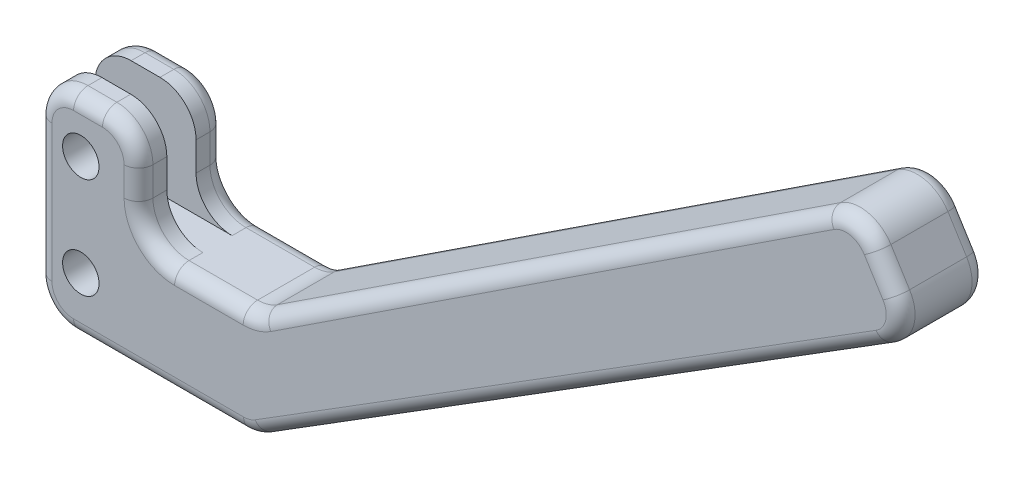
SolidWorks part; units mm, degrees
material "S316"
ref_plane "Front Plane" through (0, 0, 0) normal (0, 0, 1) x (1, 0, 0)
ref_plane "Top Plane" through (0, 0, 0) normal (0, 1, 0) x (1, 0, 0)
ref_plane "Right Plane" through (0, 0, 0) normal (1, 0, 0) x (0, 0, -1)
sketch "Sketch1" plane through (0, 0, 0) normal (0, 0, 1) x (1, 0, 0)
  line L1 (-15, 7.5) -> (15, 7.5)
  line L2 (-15, 7.5) -> (-15, -7.5)
  line L3 (-15, -7.5) -> (15, -7.5)
  line L4 (15, 7.5) -> (15, -7.5)
  line L5 (-15, 7.5) -> (15, -7.5) construction
  line L6 (-15, -7.5) -> (15, 7.5) construction
  point P0 (0, 0)
  dimension "D1" = 15
  dimension "D2" = 30
extrude "Boss-Extrude1" add sketch "Sketch1" along normal blind 11.9
sketch "Sketch2" plane through (0, 0, 11.9) normal (0, 0, 1) x (1, 0, 0)
  line L1 (-15, 7.5) -> (-1, 7.5)
  line L2 (-15, 7.5) -> (-15, 21.5)
  line L3 (-15, 21.5) -> (-1, 21.5)
  line L4 (-1, 7.5) -> (-1, 21.5)
  dimension "D1" = 14
  dimension "D2" = 14
extrude "Boss-Extrude2" add sketch "Sketch2" against normal up to surface (11.9 mm away) up to face at (0, 0, 0)
sketch "Sketch3" plane through (0, 0, 11.9) normal (0, 0, 1) x (1, 0, 0)
  line L0 (-15, -7.5) -> (15, -7.5) construction
  line L1 (-15, 21.5) -> (-15, -7.5) construction
  circle A0 centre (-9, 0.5) radius 2.525
  circle A1 centre (-9, 14.5) radius 1.65
  dimension "D1" = 5.05
  dimension "D6" = 3.3
  dimension "D2" = 8
  dimension "D3" = 6
  dimension "D4" = 6
  dimension "D5" = 14
extrude "Cut-Extrude2" cut sketch "Sketch3" against normal up to surface (11.9 mm away) up to face at (-0.3333, 7.1667, 0)
sketch "Sketch4" plane through (0, 0, 11.9) normal (0, 0, 1) x (1, 0, 0)
  line L0 (15, -7.5) -> (106.5237, 49.6904)
  line L1 (106.5237, 49.6904) -> (98.5749, 62.4111)
  line L2 (98.5749, 62.4111) -> (15, 7.5)
  line L3 (15, 7.5) -> (15, -7.5)
  dimension "D1" = 15
  dimension "D2" = 58
  dimension "D3" = 100
extrude "Boss-Extrude3" add sketch "Sketch4" against normal up to surface (11.9 mm away) up to face at (-6.475, 0.5, 0)
sketch "Sketch5" plane through (0, 7.5, 0) normal (0, 1, 0) x (1, 0, 0)
  line L0 (-15, -5.95) -> (-1, -5.95) construction
  line L1 (-15, 0) -> (-15, -11.9) construction
  line L2 (-1, 0) -> (-1, -11.9) construction
  line L4 (-1, -7.975) -> (-15, -7.975)
  line L5 (-1, -7.975) -> (-1, -3.925)
  line L6 (-1, -3.925) -> (-15, -3.925)
  line L7 (-15, -7.975) -> (-15, -3.925)
  line L8 (-1, -7.975) -> (-15, -3.925) construction
  line L9 (-1, -3.925) -> (-15, -7.975) construction
  point P6 (-8, -5.95)
  dimension "D1" = 4.05
extrude "Cut-Extrude3" cut sketch "Sketch5" along normal blind 26
fillet "Fillet1" radius 5 11 edges at (98.5749, 62.4111, 5.95) (106.5237, 49.6904, 5.95) (15, -7.5, 5.95) (-15, -7.5, 5.95) (15, 7.5, 5.95) (-1, 7.5, 9.9375) (-1, 7.5, 1.9625) (-1, 21.5, 9.9375) (-1, 21.5, 1.9625) (-15, 21.5, 9.9375) (-15, 21.5, 1.9625)
fillet "Fillet2" radius 2 32 edges at (14.9445, -7.3063, 11.9) (1.7831, -7.5, 11.9) (-13.5355, -6.0355, 11.9) (-15, 7, 11.9) (-13.5355, 20.0355, 11.9) (-8, 21.5, 11.9) (-2.4645, 20.0355, 11.9) (-1, 14.5, 11.9) (0.4645, 8.9645, 11.9) (8.7522, 7.5, 11.9) (14.9373, 7.7097, 11.9) (55.2749, 33.9617, 11.9) (55.2749, 33.9617, 0) (98.1146, 60.3078, 11.9) (102.5799, 56.0018, 0) (102.5799, 56.0018, 11.9) (104.5057, 50.1563, 11.9) (14.9373, 7.7097, 0) (8.7522, 7.5, 0) (0.4645, 8.9645, 0) (-1, 14.5, 0) (-2.4645, 20.0355, 0) (-8, 21.5, 0) (-13.5355, 20.0355, 0) (-15, 7, 0) (-13.5355, -6.0355, 0) (1.7831, -7.5, 0) (14.9445, -7.3063, 0) (59.2497, 20.1503, 0) (59.2497, 20.1503, 11.9) (104.5057, 50.1563, 0) (98.1146, 60.3078, 0)
sketch "Sketch6" plane through (0, 0, 11.9) normal (0, 0, 1) x (1, 0, 0)
  circle A0 centre (-9, 14.5) radius 2.525
  dimension "D1" = 5.05
extrude "Cut-Extrude4" cut sketch "Sketch6" against normal up to surface (3.925 mm away) up to face at (-6.4336, 14.9336, 7.975)
